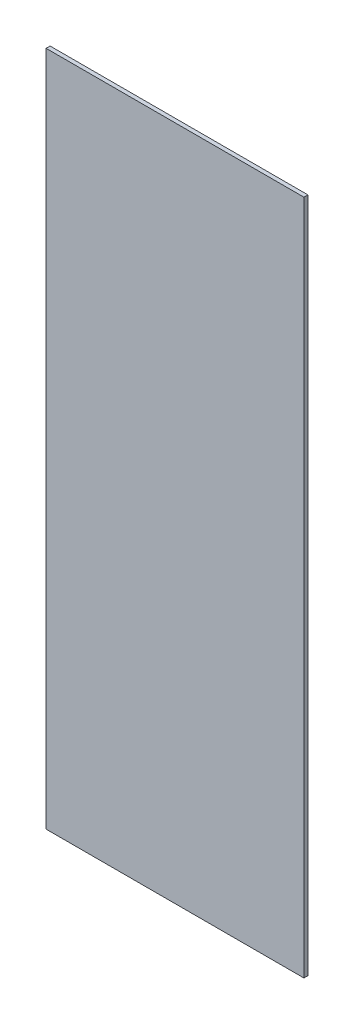
SolidWorks part; units mm, degrees
material "PMMA(有机玻璃)"
ref_plane "前视" through (0, 0, 0) normal (0, 0, 1) x (1, 0, 0)
ref_plane "上视" through (0, 0, 0) normal (0, 1, 0) x (1, 0, 0)
ref_plane "右视" through (0, 0, 0) normal (1, 0, 0) x (0, 0, -1)
sketch "草图1" plane through (0, 0, 0) normal (0, 0, 1) x (1, 0, 0)
  line L1 (-160.5, 421) -> (160.5, 421)
  line L2 (-160.5, 421) -> (-160.5, -421)
  line L3 (-160.5, -421) -> (160.5, -421)
  line L4 (160.5, 421) -> (160.5, -421)
  line L5 (-160.5, 421) -> (160.5, -421) construction
  line L6 (-160.5, -421) -> (160.5, 421) construction
  point P0 (0, 0)
  dimension "D1" = 842
  dimension "D2" = 321
extrude "凸台-拉伸1" add sketch "草图1" along normal blind 5
hole_wizard "M5 间隙孔1" positions "草图3" profile "草图2" hole size "M5" standard "GB"
sketch "草图3" plane through (0, 0, 5) normal (0, 0, 1) x (1, 0, 0)
  line L0 (-427.5, 273) -> (-427.5, -273) construction
  line L1 (-427.5, -273) -> (427.5, -273) construction
  line L2 (0, 273) -> (0, -273) construction
  line L3 (427.5, 273) -> (-427.5, 273) construction
  line L5 (-427.5, 0) -> (427.5, 0) construction
  line L6 (427.5, -273) -> (427.5, 273) construction
  point P0 (-375, -261)
  point P46 (415.5, 250)
  point P48 (-415.5, 250)
  point P58 (-125, -261)
  point P59 (125, -261)
  point P61 (-125, 261)
  point P62 (125, 261)
  point P64 (-375, 261)
  point P88 (375, -261)
  point P89 (375, 261)
  point P108 (415.5, 0)
  point P109 (-415.5, 0)
  point P110 (415.5, -250)
  point P111 (-415.5, -250)
  dimension "D1" = 12
  dimension "D2" = 12
  dimension "D5" = 3
  dimension "D3" = 12
  dimension "D6" = 4
  dimension "D4" = 2
sketch "草图2" plane through (-375, -261, 5) normal (1, 0, 0) x (0, -1, 0)
  line L0 (0, 0) -> (0, 5)
  line L1 (0, 5) -> (2.75, 5)
  line L2 (2.75, 5) -> (2.75, 0)
  line L5 (2.75, 0) -> (0, 0)
  line L11 (0, -6.35) -> (0, 107.95) construction
  dimension "通孔孔直径" = 5.5
  dimension "通孔孔深度" = 5
